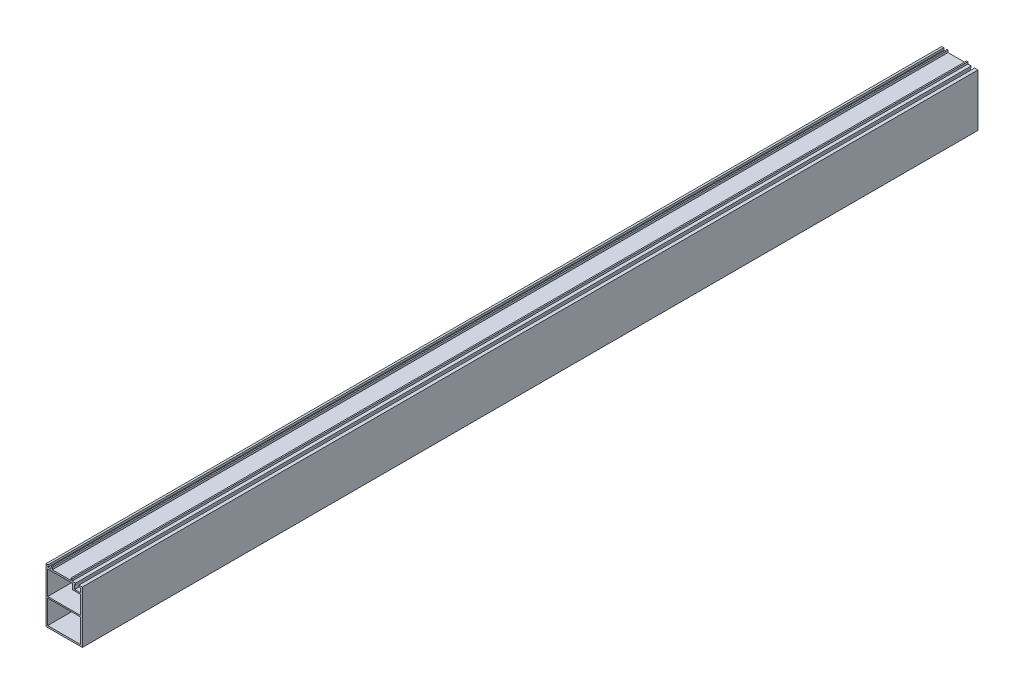
SolidWorks part; units mm, degrees
ref_plane "Front Plane" through (0, 0, 0) normal (0, 0, 1) x (1, 0, 0)
ref_plane "Top Plane" through (0, 0, 0) normal (0, 1, 0) x (1, 0, 0)
ref_plane "Right Plane" through (0, 0, 0) normal (1, 0, 0) x (0, 0, -1)
sketch "Sketch1" plane through (0, 0, 0) normal (0, 0, 1) x (1, 0, 0)
  line L0 (21.5, 0) -> (-21.5, 0) construction
  line L1 (19.5, 0.8) -> (-19.5, 0.8)
  line L2 (19.5, -0.8) -> (-19.5, -0.8)
  line L3 (19.5, -29) -> (19.5, -0.8)
  line L4 (21.5, -31) -> (-21.5, -31)
  line L5 (21.5, -31) -> (21.5, 31)
  line L6 (21.5, 31) -> (17.5, 31)
  line L7 (-21.5, -31) -> (-21.5, 31)
  line L8 (21.5, -31) -> (-21.5, 31) construction
  line L9 (21.5, 31) -> (-21.5, -31) construction
  line L10 (19.5, 29) -> (17.5, 29)
  line L11 (-19.5, -29) -> (-19.5, -0.8)
  line L12 (19.5, -29) -> (-19.5, -29)
  line L13 (40.5035, 0.8) -> (-40.5035, 0.8) construction
  line L14 (40.5035, -0.8) -> (-40.5035, -0.8) construction
  line L15 (40.5035, 0) -> (-40.5035, 0) construction
  line L16 (-19.5, 0.8) -> (-19.5, 29)
  line L17 (-19.5, -29) -> (-19.5, 29) construction
  line L18 (19.5, 0.8) -> (19.5, 22.4)
  line L19 (19.5, -29) -> (19.5, 29) construction
  line L20 (13.5, 31) -> (13.5, 29)
  line L21 (17.5, 31) -> (17.5, 29)
  line L22 (13.5, 31) -> (9.5, 31)
  line L23 (21.5, 31) -> (-21.5, 31) construction
  line L24 (13.5, 29) -> (12.5, 29)
  line L25 (19.5, 29) -> (-19.5, 29) construction
  line L26 (12.5, 29) -> (12.5, 24)
  line L27 (12.5, 24) -> (19.5, 24)
  line L28 (10.1, 29) -> (10.1, 22.4)
  line L29 (10.1, 22.4) -> (19.5, 22.4)
  line L30 (19.5, 24) -> (19.5, 29)
  line L31 (10.1, 29) -> (-19.5, 29)
  line L32 (-19, 31) -> (-19, 33.5)
  line L33 (-19, 33.5) -> (-21.5, 33.5)
  line L34 (-21.5, 33.5) -> (-21.5, 31)
  line L35 (-15.5, 33.5) -> (-15.5, 31)
  line L36 (-15.5, 33.5) -> (-14, 33.5)
  line L37 (-14, 33.5) -> (-14, 31)
  line L38 (8, 33.5) -> (8, 31)
  line L39 (8, 33.5) -> (9.5, 33.5)
  line L40 (9.5, 33.5) -> (9.5, 31)
  line L41 (8, 31) -> (-14, 31)
  line L42 (-15.5, 31) -> (-19, 31)
  point P4 (0, 0)
  point P9 (0, 0)
  dimension "D1" = 0.8
  dimension "D3" = 43
  dimension "D4" = 62
  dimension "D6" = 4
  dimension "D7" = 4
  dimension "D8" = 1.6
  dimension "D9" = 5
  dimension "D10" = 7
  dimension "D11" = 2.4
  dimension "D12" = 2.5
  dimension "D13" = 1.5
  dimension "D14" = 1.5
  dimension "D15" = 22
  dimension "D16" = 3.5
  dimension "D17" = 2.5
  dimension "D2" = 0.8
  dimension "D5" = 2
extrude "Boss-Extrude1" add sketch "Sketch1" along normal mid plane 1060
